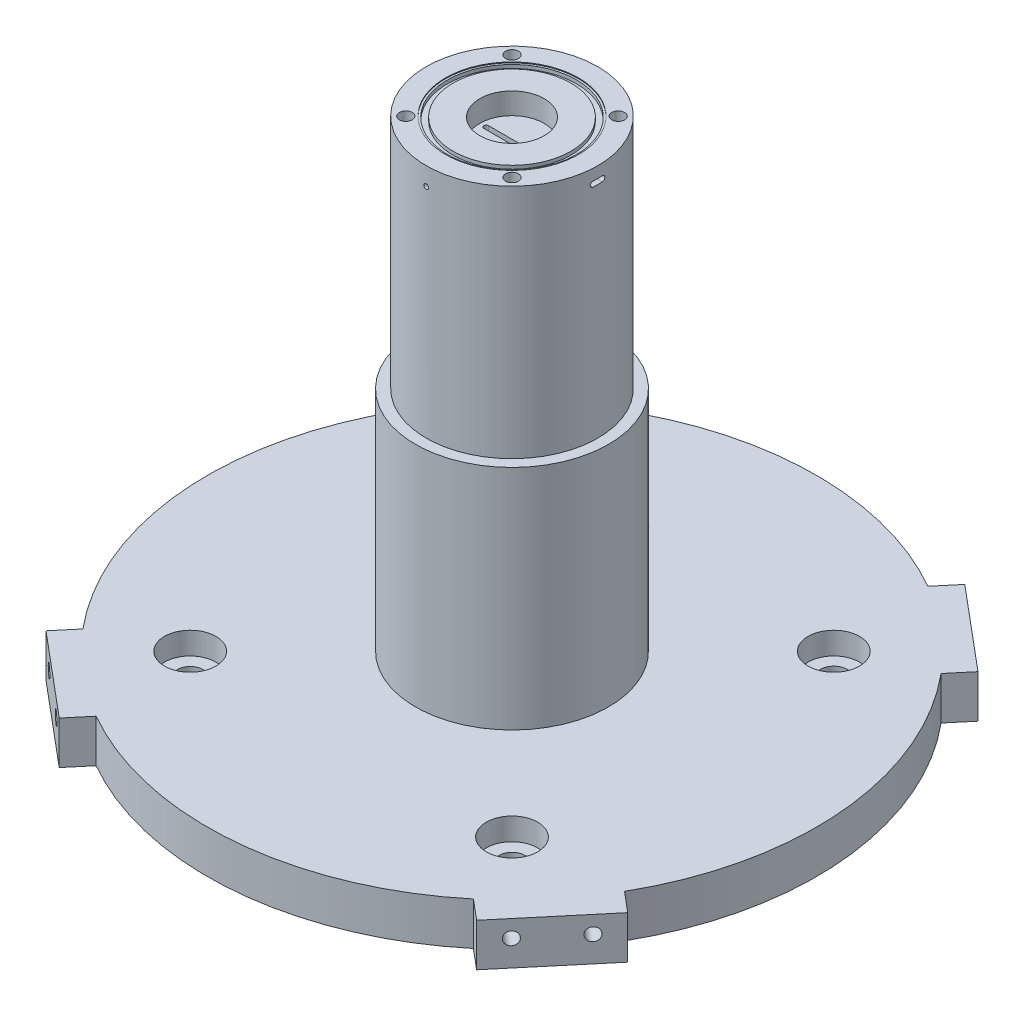
from build123d import *

# Parameters (mm, degrees)
SKETCH4_R           = 7.5
CUT_EXTRUDE1_DEPTH  = 5
SKETCH8_R           = 1.5
CUT_EXTRUDE6_DEPTH  = 3
CUT_EXTRUDE15_DEPTH = 8
CUT_EXTRUDE8_START  = 8
CUT_EXTRUDE8_DEPTH  = 8
BOSS_EXTRUDE3_START = 71
SKETCH16_W          = 10
SKETCH16_H          = 25
BOSS_EXTRUDE3_DEPTH = 5
SKETCH17_R          = 1.5
CUT_EXTRUDE10_DEPTH = 5
CIRPATTERN2_COUNT   = 4
SKETCH21_R          = 3.1
SKETCH21_R_2        = 3
CUT_EXTRUDE12_DEPTH = 155.938697631
SKETCH22_R          = 6
CUT_EXTRUDE13_DEPTH = 5.2
SKETCH25_R          = 0.55
CUT_EXTRUDE16_DEPTH = 6
CUT_EXTRUDE17_START = -6
SKETCH27_R          = 0.55
CUT_EXTRUDE17_DEPTH = 6
CUT_EXTRUDE19_DEPTH = 1.1


with BuildPart() as part:
    # Sketch1 → Revolve1 (revolve)
    with BuildSketch(Plane.XY, mode=Mode.PRIVATE) as revolve1_sk:
        Polygon((22.5, 0), (22.5, 53), (20, 53), (20, 108), (0, 108), (0, 0), (0, -10), (71, -10), (71, 0), align=None)
    revolve(revolve1_sk.sketch.rotate(Axis((0, 0, 0), (0, 1, 0)), 90), axis=Axis((0, 0, 0), (0, 1, 0)))

    # Sketch3 → Cut-Revolve1 (revolve, cut)
    with BuildSketch(Plane.XY, mode=Mode.PRIVATE) as cut_revolve1_sk:
        Polygon((0, 108), (0, 107.8), (13.75, 107.8), (13.75, 107), (15.05, 107), (15.05, 107.8), (15.5, 107.8), (15.5, 108), align=None)
    revolve(cut_revolve1_sk.sketch.rotate(Axis((0, -12.550098123, 0), (0, 1, 0)), 90), axis=Axis((0, -12.550098123, 0), (0, 1, 0)), mode=Mode.SUBTRACT)

    # Sketch4 → Cut-Extrude1 (cut)
    with BuildSketch(Plane(origin=(0, 107.8, 0), x_dir=(1, 0, 0), z_dir=(0, 1, 0))):
        with Locations(Location((0, 0, 0), (0, 0, 270))):
            Circle(SKETCH4_R)
    extrude(amount=-CUT_EXTRUDE1_DEPTH, mode=Mode.SUBTRACT)

    # Sketch8 → Cut-Extrude6 (cut, symmetric)
    with BuildSketch(Plane(origin=(0, 107.8, 0), x_dir=(1, 0, 0), z_dir=(0, 1, 0))):
        with Locations(Location((12.374368671, 12.374368671, 0), (0, 0, 270))):
            Circle(SKETCH8_R)
        with Locations(Location((12.374368671, -12.374368671, 0), (0, 0, 270))):
            Circle(SKETCH8_R)
        with Locations(Location((-12.374368671, -12.374368671, 0), (0, 0, 270))):
            Circle(SKETCH8_R)
        with Locations(Location((-12.374368671, 12.374368671, 0), (0, 0, 270))):
            Circle(SKETCH8_R)
    extrude(amount=CUT_EXTRUDE6_DEPTH, both=True, mode=Mode.SUBTRACT)

    # Sketch24 → Cut-Extrude15 (cut)
    with BuildSketch(Plane(origin=(20, 0, 0), x_dir=(0, 0, -1), z_dir=(1, 0, 0))):
        with BuildLine():
            Line((-1.1, 105.4), (1.1, 105.4))
            ThreePointArc((1.1, 105.4), (1.7, 104.8), (1.1, 104.2))
            Line((1.1, 104.2), (-1.1, 104.2))
            ThreePointArc((-1.1, 104.2), (-1.7, 104.8), (-1.1, 105.4))
        make_face()
    extrude(amount=-CUT_EXTRUDE15_DEPTH, mode=Mode.SUBTRACT)

    # Sketch10 → Cut-Extrude8 (cut)
    with BuildSketch(Plane(origin=(-20, 0, 0), x_dir=(0, 0, -1), z_dir=(1, 0, 0)).offset(CUT_EXTRUDE8_START)):
        with BuildLine():
            Line((1.1, 104.2), (-1.1, 104.2))
            ThreePointArc((-1.1, 104.2), (-1.7, 104.8), (-1.1, 105.4))
            Line((-1.1, 105.4), (1.1, 105.4))
            ThreePointArc((1.1, 105.4), (1.7, 104.8), (1.1, 104.2))
        make_face()
    extrude(amount=-CUT_EXTRUDE8_DEPTH, mode=Mode.SUBTRACT)

    # Sketch16 → Boss-Extrude3 (add, symmetric)
    with BuildSketch(Plane(origin=(0, 0, 0), x_dir=(0, -1, 0), z_dir=(-0.6427876096865403, 0, 0.7660444431189772)).offset(BOSS_EXTRUDE3_START)):
        with Locations((5, 0)):
            Rectangle(SKETCH16_W, SKETCH16_H)
    boss_extrude3 = extrude(amount=BOSS_EXTRUDE3_DEPTH, both=True)

    # Sketch17 → Cut-Extrude10 (cut)
    with BuildSketch(Plane(origin=(-48.851858336, 0, 58.219377677), x_dir=(0.7660444431189771, 0, 0.6427876096865404), z_dir=(-0.6427876096865404, 0, 0.7660444431189771))):
        with Locations((6.75, -4)):
            Circle(SKETCH17_R)
        with Locations((-6.75, -4)):
            Circle(SKETCH17_R)
    cut_extrude10 = extrude(amount=-CUT_EXTRUDE10_DEPTH, mode=Mode.SUBTRACT)

    # CirPattern2: Boss-Extrude3, Cut-Extrude10 ×4 about axis
    cirpattern2_axis = Axis((0, 0, 0), (0, 1, 0))
    add([boss_extrude3.rotate(cirpattern2_axis, i * 360 / CIRPATTERN2_COUNT) for i in range(1, CIRPATTERN2_COUNT)])
    add([cut_extrude10.rotate(cirpattern2_axis, i * 360 / CIRPATTERN2_COUNT) for i in range(1, CIRPATTERN2_COUNT)], mode=Mode.SUBTRACT)

    # Sketch21 → Cut-Extrude12 (cut, through all)
    with BuildSketch(Plane(origin=(0, -10, 0), x_dir=(-1, 0, 0), z_dir=(0, -1, 0))):
        with Locations(Location((-37.5, 37.5, 0), (0, 0, 90))):
            Circle(SKETCH21_R)
        with Locations(Location((37.5, 37.5, 0), (0, 0, 90))):
            Circle(SKETCH21_R_2)
        with Locations(Location((-37.5, -37.5, 0), (0, 0, 90))):
            Circle(SKETCH21_R_2)
        with Locations(Location((37.5, -37.5, 0), (0, 0, 90))):
            Circle(SKETCH21_R_2)
    extrude(amount=-CUT_EXTRUDE12_DEPTH, mode=Mode.SUBTRACT)

    # Sketch22 → Cut-Extrude13 (cut)
    with BuildSketch(Plane(origin=(0, 0, 0), x_dir=(1, 0, 0), z_dir=(0, 1, 0))):
        with Locations(Location((-37.5, 37.5, 0), (0, 0, 270))):
            Circle(SKETCH22_R)
        with Locations(Location((37.5, 37.5, 0), (0, 0, 270))):
            Circle(SKETCH22_R)
        with Locations(Location((-37.5, -37.5, 0), (0, 0, 270))):
            Circle(SKETCH22_R)
        with Locations(Location((37.5, -37.5, 0), (0, 0, 270))):
            Circle(SKETCH22_R)
    extrude(amount=-CUT_EXTRUDE13_DEPTH, mode=Mode.SUBTRACT)

    # Sketch25 → Cut-Extrude16 (cut)
    with BuildSketch(Plane(origin=(0, 0, -20), x_dir=(-1, 0, 0), z_dir=(0, 0, -1))):
        with Locations((0, 103.8)):
            Circle(SKETCH25_R)
    extrude(amount=-CUT_EXTRUDE16_DEPTH, mode=Mode.SUBTRACT)

    # Sketch27 → Cut-Extrude17 (cut)
    with BuildSketch(Plane.XY.offset(20).offset(CUT_EXTRUDE17_START)):
        with Locations(Location((0, 103.8, 0), (0, 0, 180))):
            Circle(SKETCH27_R)
    extrude(amount=CUT_EXTRUDE17_DEPTH, mode=Mode.SUBTRACT)

    # Sketch28 → Cut-Extrude19 (cut)
    with BuildSketch(Plane(origin=(0, 102.8, 0), x_dir=(1, 0, 0), z_dir=(0, 1, 0))):
        with BuildLine():
            Line((-6, 0.55), (6, 0.55))
            ThreePointArc((6, 0.55), (6.55, 0), (6, -0.55))
            Line((6, -0.55), (-6, -0.55))
            ThreePointArc((-6, -0.55), (-6.55, 0), (-6, 0.55))
        make_face()
    extrude(amount=-CUT_EXTRUDE19_DEPTH, mode=Mode.SUBTRACT)


solid = part.part
